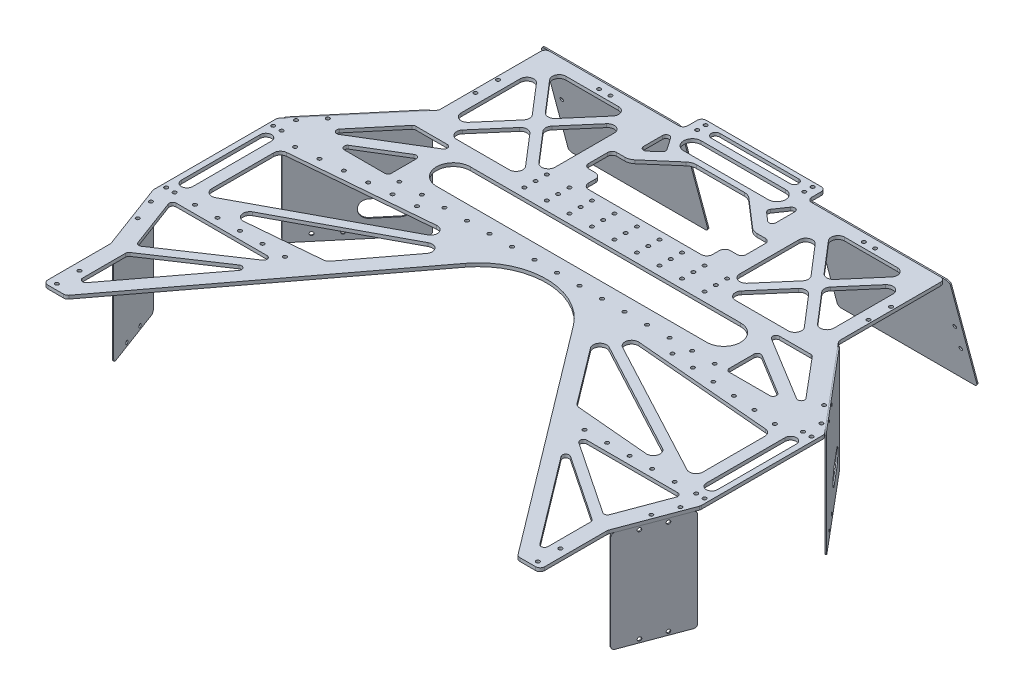
from build123d import *

# Parameters (mm, degrees)
SKETCH_1_R           = 1.6
EXTRUDE_1_DEPTH      = 3
SKETCH_2_W           = 60
SKETCH_2_H           = 90
SKETCH_2_R           = 1.6
EXTRUDE_2_DEPTH      = 1
SKETCH_3_W           = 95
SKETCH_3_H           = 96
SKETCH_3_R           = 1.6
EXTRUDE_3_DEPTH      = 1
EXTRUDE_5_DEPTH      = 4
EXTRUDE_5_DEPTH_BACK = 120
SKETCH_7_R           = 1.6
CUT_EXTRUDE_2_DEPTH  = 1
FILLET_1_R           = 3
FILLET_2_R           = 3
FILLET_3_R           = 3
CUT_EXTRUDE_4_DEPTH  = 10
CUT_EXTRUDE_1_DEPTH  = 10
CUT_EXTRUDE_3_DEPTH  = 10
FILLET_4_R           = 4
SKETCH_10_R          = 1.6
CUT_EXTRUDE_5_DEPTH  = 10


with BuildPart() as part:
    # 草图1 → 凸台-拉伸1 (new body)
    with BuildSketch(Plane(origin=(0, 0, 0), x_dir=(1, 0, 0), z_dir=(0, 1, 0))):
        with BuildLine():
            Line((-55, 0), (55, 0))
            Line((55, 0), (55, -16.419274896))
            Line((55, -16.419274896), (177.5, -16.419274896))
            Line((177.5, -16.419274896), (177.5, -111))
            Line((177.5, -111), (243, -189))
            Line((243, -189), (243, -299))
            Line((243, -299), (220.55, -359))
            Line((220.55, -359), (220.55, -419))
            Line((220.55, -419), (200.55, -419))
            Line((200.55, -419), (47.880319216, -216.840975791))
            ThreePointArc((47.880319216, -216.840975791), (0, -193), (-47.880319216, -216.840975791))
            Line((-47.880319216, -216.840975791), (-200.55, -419))
            Line((-200.55, -419), (-220.55, -419))
            Line((-220.55, -419), (-220.55, -359))
            Line((-220.55, -359), (-243, -299))
            Line((-243, -299), (-243, -189))
            Line((-243, -189), (-177.5, -111))
            Line((-177.5, -111), (-177.5, -16.419274896))
            Line((-177.5, -16.419274896), (-55, -16.419274896))
            Line((-55, -16.419274896), (-55, 0))
        make_face()
        with Locations(Location((47.5, -4, 0), (0, 0, 270))):
            Circle(SKETCH_1_R, mode=Mode.SUBTRACT)
        with Locations(Location((-47.5, -4, 0), (0, 0, 90))):
            Circle(SKETCH_1_R, mode=Mode.SUBTRACT)
        with Locations(Location((47.5, -11.5, 0), (0, 0, 270))):
            Circle(SKETCH_1_R, mode=Mode.SUBTRACT)
        with Locations(Location((-47.5, -11.5, 0), (0, 0, 90))):
            Circle(SKETCH_1_R, mode=Mode.SUBTRACT)
        with Locations(Location((231.5, -196.5, 0), (0, 0, 270))):
            Circle(SKETCH_1_R, mode=Mode.SUBTRACT)
        with Locations(Location((-231.5, -196.5, 0), (0, 0, 90))):
            Circle(SKETCH_1_R, mode=Mode.SUBTRACT)
        with Locations(Location((239, -196.5, 0), (0, 0, 270))):
            Circle(SKETCH_1_R, mode=Mode.SUBTRACT)
        with Locations(Location((-239, -196.5, 0), (0, 0, 90))):
            Circle(SKETCH_1_R, mode=Mode.SUBTRACT)
        with Locations(Location((231.5, -291.5, 0), (0, 0, 270))):
            Circle(SKETCH_1_R, mode=Mode.SUBTRACT)
        with Locations(Location((-231.5, -291.5, 0), (0, 0, 90))):
            Circle(SKETCH_1_R, mode=Mode.SUBTRACT)
        with Locations(Location((239, -291.5, 0), (0, 0, 270))):
            Circle(SKETCH_1_R, mode=Mode.SUBTRACT)
        with Locations(Location((-239, -291.5, 0), (0, 0, 90))):
            Circle(SKETCH_1_R, mode=Mode.SUBTRACT)
        with Locations(Location((213.55, -394, 0), (0, 0, 270))):
            Circle(SKETCH_1_R, mode=Mode.SUBTRACT)
        with Locations(Location((-213.55, -394, 0), (0, 0, 90))):
            Circle(SKETCH_1_R, mode=Mode.SUBTRACT)
        with Locations(Location((213.55, -414, 0), (0, 0, 270))):
            Circle(SKETCH_1_R, mode=Mode.SUBTRACT)
        with Locations(Location((-213.55, -414, 0), (0, 0, 90))):
            Circle(SKETCH_1_R, mode=Mode.SUBTRACT)
        with Locations(Location((234.987500732, -309, 0), (0, 0, 270))):
            Circle(SKETCH_1_R, mode=Mode.SUBTRACT)
        with Locations(Location((227.978719043, -327.731710526, 0), (0, 0, 270))):
            Circle(SKETCH_1_R, mode=Mode.SUBTRACT)
        with Locations(Location((-227.978719043, -327.731710526, 0), (0, 0, 90))):
            Circle(SKETCH_1_R, mode=Mode.SUBTRACT)
        with Locations(Location((-234.987500732, -309, 0), (0, 0, 90))):
            Circle(SKETCH_1_R, mode=Mode.SUBTRACT)
        with Locations(Location((220.342791881, -166.683968756, 0), (0, 0, 270))):
            Circle(SKETCH_1_R, mode=Mode.SUBTRACT)
        with Locations(Location((233.204330939, -182, 0), (0, 0, 270))):
            Circle(SKETCH_1_R, mode=Mode.SUBTRACT)
        with Locations(Location((-233.204330939, -182, 0), (0, 0, 90))):
            Circle(SKETCH_1_R, mode=Mode.SUBTRACT)
        with Locations(Location((-220.342791881, -166.683968756, 0), (0, 0, 90))):
            Circle(SKETCH_1_R, mode=Mode.SUBTRACT)
        with Locations(Location((112.5, -23.615427319, 0), (0, 0, 270))):
            Circle(SKETCH_1_R, mode=Mode.SUBTRACT)
        with Locations(Location((122.5, -23.615427319, 0), (0, 0, 270))):
            Circle(SKETCH_1_R, mode=Mode.SUBTRACT)
        with Locations(Location((-122.5, -23.615427319, 0), (0, 0, 90))):
            Circle(SKETCH_1_R, mode=Mode.SUBTRACT)
        with Locations(Location((-112.5, -23.615427319, 0), (0, 0, 90))):
            Circle(SKETCH_1_R, mode=Mode.SUBTRACT)
        with Locations(Location((174.5, -61.419274896, 0), (0, 0, 270))):
            Circle(SKETCH_1_R, mode=Mode.SUBTRACT)
        with Locations(Location((174.5, -81.419274896, 0), (0, 0, 270))):
            Circle(SKETCH_1_R, mode=Mode.SUBTRACT)
        with Locations(Location((-174.5, -81.419274896, 0), (0, 0, 90))):
            Circle(SKETCH_1_R, mode=Mode.SUBTRACT)
        with Locations(Location((-174.5, -61.419274896, 0), (0, 0, 90))):
            Circle(SKETCH_1_R, mode=Mode.SUBTRACT)
    extrude(amount=EXTRUDE_1_DEPTH)

    # 草图4 → 切除-拉伸1 (cut)
    with BuildSketch(Plane(origin=(0, 3, 0), x_dir=(1, 0, 0), z_dir=(0, 1, 0))):
        with BuildLine():
            Line((-50, -105.5), (50, -105.5))
            ThreePointArc((50, -105.5), (53.535533906, -104.035533906), (55, -100.5))
            Line((55, -100.5), (55, -94.5))
            ThreePointArc((55, -94.5), (56.464466094, -90.964466094), (60, -89.5))
            Line((60, -89.5), (66, -89.5))
            ThreePointArc((66, -89.5), (68.828427125, -88.328427125), (70, -85.5))
            Line((70, -85.5), (70, -68.5))
            ThreePointArc((70, -68.5), (68.828427125, -65.671572875), (66, -64.5))
            Line((66, -64.5), (58.730333263, -64.5))
            ThreePointArc((58.730333263, -64.5), (55.235258748, -63.869335843), (52.181027878, -62.056890828))
            Line((52.181027878, -62.056890828), (27.818972122, -40.943109172))
            ThreePointArc((27.818972122, -40.943109172), (24.764741252, -39.130664157), (21.269666737, -38.5))
            Line((21.269666737, -38.5), (-21.269666737, -38.5))
            ThreePointArc((-21.269666737, -38.5), (-24.764741252, -39.130664157), (-27.818972122, -40.943109172))
            Line((-27.818972122, -40.943109172), (-52.181027878, -62.056890828))
            ThreePointArc((-52.181027878, -62.056890828), (-55.235258748, -63.869335843), (-58.730333263, -64.5))
            Line((-58.730333263, -64.5), (-66, -64.5))
            ThreePointArc((-66, -64.5), (-68.828427125, -65.671572875), (-70, -68.5))
            Line((-70, -68.5), (-70, -85.5))
            ThreePointArc((-70, -85.5), (-68.828427125, -88.328427125), (-66, -89.5))
            Line((-66, -89.5), (-60, -89.5))
            ThreePointArc((-60, -89.5), (-56.464466094, -90.964466094), (-55, -94.5))
            Line((-55, -94.5), (-55, -100.5))
            ThreePointArc((-55, -100.5), (-53.535533906, -104.035533906), (-50, -105.5))
        make_face()
    extrude(amount=-CUT_EXTRUDE_1_DEPTH, mode=Mode.SUBTRACT)

    # 草图8 → 切除-拉伸3 (cut)
    with BuildSketch(Plane(origin=(0, 3, 0), x_dir=(1, 0, 0), z_dir=(0, 1, 0))):
        with BuildLine():
            Line((238, -209), (238, -279))
            ThreePointArc((238, -279), (233, -284), (228, -279))
            Line((228, -279), (228, -209))
            ThreePointArc((228, -209), (233, -204), (238, -209))
        make_face()
        with BuildLine():
            Line((-238, -209), (-238, -279))
            ThreePointArc((-238, -279), (-233, -284), (-228, -279))
            Line((-228, -279), (-228, -209))
            ThreePointArc((-228, -209), (-233, -204), (-238, -209))
        make_face()
        with BuildLine():
            Line((206.55, -398.082426617), (206.55, -360.028410476))
            ThreePointArc((206.55, -360.028410476), (206.196356405, -358.615329524), (205.21880148, -357.535399923))
            Line((205.21880148, -357.535399923), (147.100440737, -318.631430456))
            ThreePointArc((147.100440737, -318.631430456), (143.250801795, -319.064356553), (143.037623296, -322.932392219))
            Line((143.037623296, -322.932392219), (201.155984039, -399.890377828))
            ThreePointArc((201.155984039, -399.890377828), (204.503402359, -400.926899141), (206.55, -398.082426617))
        make_face()
        with BuildLine():
            Line((-206.55, -398.082426617), (-206.55, -360.028410476))
            ThreePointArc((-206.55, -360.028410476), (-206.196356405, -358.615329524), (-205.21880148, -357.535399923))
            Line((-205.21880148, -357.535399923), (-147.100440737, -318.631430456))
            ThreePointArc((-147.100440737, -318.631430456), (-143.250801795, -319.064356553), (-143.037623296, -322.932392219))
            Line((-143.037623296, -322.932392219), (-201.155984039, -399.890377828))
            ThreePointArc((-201.155984039, -399.890377828), (-204.503402359, -400.926899141), (-206.55, -398.082426617))
        make_face()
        with BuildLine():
            Line((209.318721671, -346.213334716), (225.468509872, -303.051317253))
            ThreePointArc((225.468509872, -303.051317253), (225.123905596, -300.290314614), (222.658753293, -299))
            Line((222.658753293, -299), (142.029537012, -299))
            ThreePointArc((142.029537012, -299), (139.159081329, -301.127942565), (140.360735532, -304.493010553))
            Line((140.360735532, -304.493010553), (204.840163612, -347.655028016))
            ThreePointArc((204.840163612, -347.655028016), (207.428239005, -348.017702227), (209.318721671, -346.213334716))
        make_face()
        with BuildLine():
            Line((-209.318721671, -346.213334716), (-225.468509872, -303.051317253))
            ThreePointArc((-225.468509872, -303.051317253), (-225.123905596, -300.290314614), (-222.658753293, -299))
            Line((-222.658753293, -299), (-142.029537012, -299))
            ThreePointArc((-142.029537012, -299), (-139.159081329, -301.127942565), (-140.360735532, -304.493010553))
            Line((-140.360735532, -304.493010553), (-204.840163612, -347.655028016))
            ThreePointArc((-204.840163612, -347.655028016), (-207.428239005, -348.017702227), (-209.318721671, -346.213334716))
        make_face()
        with BuildLine():
            Line((-35, -4), (35, -4))
            ThreePointArc((35, -4), (38.75, -7.75), (35, -11.5))
            Line((35, -11.5), (-35, -11.5))
            ThreePointArc((-35, -11.5), (-38.75, -7.75), (-35, -4))
        make_face()
        with BuildLine():
            Line((-37.5, -18), (37.5, -18))
            ThreePointArc((37.5, -18), (45.25, -25.75), (37.5, -33.5))
            Line((37.5, -33.5), (-37.5, -33.5))
            ThreePointArc((-37.5, -33.5), (-45.25, -25.75), (-37.5, -18))
        make_face()
        with BuildLine():
            Line((53.262700552, -29.327417709), (45.9577168, -39.893024035))
            ThreePointArc((45.9577168, -39.893024035), (45.449090517, -41.975800238), (46.460557895, -43.866194682))
            Line((46.460557895, -43.866194682), (53.765541647, -50.1971806))
            ThreePointArc((53.765541647, -50.1971806), (56.976452269, -50.659066892), (58.730333263, -47.930113352))
            Line((58.730333263, -47.930113352), (58.730333263, -31.033521107))
            ThreePointArc((58.730333263, -31.033521107), (56.623950034, -28.169703888), (53.262700552, -29.327417709))
        make_face()
        with BuildLine():
            Line((-53.262700552, -29.327417709), (-45.9577168, -39.893024035))
            ThreePointArc((-45.9577168, -39.893024035), (-45.449090517, -41.975800238), (-46.460557895, -43.866194682))
            Line((-46.460557895, -43.866194682), (-53.765541647, -50.1971806))
            ThreePointArc((-53.765541647, -50.1971806), (-56.976452269, -50.659066892), (-58.730333263, -47.930113352))
            Line((-58.730333263, -47.930113352), (-58.730333263, -31.033521107))
            ThreePointArc((-58.730333263, -31.033521107), (-56.623950034, -28.169703888), (-53.262700552, -29.327417709))
        make_face()
        with BuildLine():
            Line((72.677992184, -226.446337249), (109.351647332, -275.008109966))
            ThreePointArc((109.351647332, -275.008109966), (111.233567595, -276.641447016), (113.616744797, -277.369375734))
            Line((113.616744797, -277.369375734), (178.57816518, -283.052763583))
            ThreePointArc((178.57816518, -283.052763583), (184.852678678, -278.784202584), (181.926242178, -271.7823384))
            Line((181.926242178, -271.7823384), (80.291166647, -217.537177833))
            ThreePointArc((80.291166647, -217.537177833), (72.90460831, -218.932552589), (72.677992184, -226.446337249))
        make_face()
        with BuildLine():
            Line((212.51341094, -211.030519833), (89.80099749, -200.491550029))
            ThreePointArc((89.80099749, -200.491550029), (83.534648252, -204.765518849), (86.462444008, -211.762800768))
            Line((86.462444008, -211.762800768), (209.174857458, -277.257459343))
            ThreePointArc((209.174857458, -277.257459343), (215.086190593, -277.109630185), (218, -271.964202348))
            Line((218, -271.964202348), (218, -217.008513577))
            ThreePointArc((218, -217.008513577), (216.420433556, -212.951449715), (212.51341094, -211.030519833))
        make_face()
        with BuildLine():
            Line((-120, -140.5), (120, -140.5))
            ThreePointArc((120, -140.5), (135, -155.5), (120, -170.5))
            Line((120, -170.5), (-120, -170.5))
            ThreePointArc((-120, -170.5), (-135, -155.5), (-120, -140.5))
        make_face()
        with BuildLine():
            Line((100.350753729, -125.5), (147.149246271, -125.5))
            ThreePointArc((147.149246271, -125.5), (152.602461969, -122.002486473), (151.698112445, -115.587479517))
            Line((151.698112445, -115.587479517), (128.298866174, -88.382499937))
            ThreePointArc((128.298866174, -88.382499937), (123.75, -86.29502042), (119.201133826, -88.382499937))
            Line((119.201133826, -88.382499937), (95.801887555, -115.587479517))
            ThreePointArc((95.801887555, -115.587479517), (94.897538031, -122.002486473), (100.350753729, -125.5))
        make_face()
        with BuildLine():
            Line((82, -103.188756541), (82, -50.730518355))
            ThreePointArc((82, -50.730518355), (85.913519356, -45.1049874), (92.548866174, -46.817997872))
            Line((92.548866174, -46.817997872), (115.108766112, -73.047116965))
            ThreePointArc((115.108766112, -73.047116965), (116.559899938, -76.959637448), (115.108766112, -80.872157931))
            Line((115.108766112, -80.872157931), (92.548866174, -107.101277025))
            ThreePointArc((92.548866174, -107.101277025), (85.913519356, -108.814287496), (82, -103.188756541))
        make_face()
        with BuildLine():
            Line((100.350753729, -28.419274896), (147.149246271, -28.419274896))
            ThreePointArc((147.149246271, -28.419274896), (152.602461969, -31.916788423), (151.698112445, -38.331795379))
            Line((151.698112445, -38.331795379), (128.298866174, -65.536774959))
            ThreePointArc((128.298866174, -65.536774959), (123.75, -67.624254476), (119.201133826, -65.536774959))
            Line((119.201133826, -65.536774959), (95.801887555, -38.331795379))
            ThreePointArc((95.801887555, -38.331795379), (94.897538031, -31.916788423), (100.350753729, -28.419274896))
        make_face()
        with BuildLine():
            Line((165.5, -103.188756541), (165.5, -50.730518355))
            ThreePointArc((165.5, -50.730518355), (161.586480644, -45.1049874), (154.951133826, -46.817997872))
            Line((154.951133826, -46.817997872), (132.391233888, -73.047116965))
            ThreePointArc((132.391233888, -73.047116965), (130.940100062, -76.959637448), (132.391233888, -80.872157931))
            Line((132.391233888, -80.872157931), (154.951133826, -107.101277025))
            ThreePointArc((154.951133826, -107.101277025), (161.586480644, -108.814287496), (165.5, -103.188756541))
        make_face()
        with BuildLine():
            Line((-132.391233888, -73.047116965), (-154.951133826, -46.817997872))
            ThreePointArc((-154.951133826, -46.817997872), (-161.586480644, -45.1049874), (-165.5, -50.730518355))
            Line((-165.5, -50.730518355), (-165.5, -103.188756541))
            ThreePointArc((-165.5, -103.188756541), (-161.586480644, -108.814287496), (-154.951133826, -107.101277025))
            Line((-154.951133826, -107.101277025), (-132.391233888, -80.872157931))
            ThreePointArc((-132.391233888, -80.872157931), (-130.940100062, -76.959637448), (-132.391233888, -73.047116965))
        make_face()
        with BuildLine():
            Line((-128.298866174, -88.382499937), (-151.698112445, -115.587479517))
            ThreePointArc((-151.698112445, -115.587479517), (-152.602461969, -122.002486473), (-147.149246271, -125.5))
            Line((-147.149246271, -125.5), (-100.350753729, -125.5))
            ThreePointArc((-100.350753729, -125.5), (-94.897538031, -122.002486473), (-95.801887555, -115.587479517))
            Line((-95.801887555, -115.587479517), (-119.201133826, -88.382499937))
            ThreePointArc((-119.201133826, -88.382499937), (-123.75, -86.29502042), (-128.298866174, -88.382499937))
        make_face()
        with BuildLine():
            Line((-128.298866174, -65.536774959), (-151.698112445, -38.331795379))
            ThreePointArc((-151.698112445, -38.331795379), (-152.602461969, -31.916788423), (-147.149246271, -28.419274896))
            Line((-147.149246271, -28.419274896), (-100.350753729, -28.419274896))
            ThreePointArc((-100.350753729, -28.419274896), (-94.897538031, -31.916788423), (-95.801887555, -38.331795379))
            Line((-95.801887555, -38.331795379), (-119.201133826, -65.536774959))
            ThreePointArc((-119.201133826, -65.536774959), (-123.75, -67.624254476), (-128.298866174, -65.536774959))
        make_face()
        with BuildLine():
            Line((-92.548866174, -107.101277025), (-115.108766112, -80.872157931))
            ThreePointArc((-115.108766112, -80.872157931), (-116.559899938, -76.959637448), (-115.108766112, -73.047116965))
            Line((-115.108766112, -73.047116965), (-92.548866174, -46.817997872))
            ThreePointArc((-92.548866174, -46.817997872), (-85.913519356, -45.1049874), (-82, -50.730518355))
            Line((-82, -50.730518355), (-82, -103.188756541))
            ThreePointArc((-82, -103.188756541), (-85.913519356, -108.814287496), (-92.548866174, -107.101277025))
        make_face()
        with BuildLine():
            Line((-218, -217.008513577), (-218, -271.964202348))
            ThreePointArc((-218, -271.964202348), (-215.086190593, -277.109630185), (-209.174857458, -277.257459343))
            Line((-209.174857458, -277.257459343), (-86.462444008, -211.762800768))
            ThreePointArc((-86.462444008, -211.762800768), (-83.534648252, -204.765518849), (-89.80099749, -200.491550029))
            Line((-89.80099749, -200.491550029), (-212.51341094, -211.030519833))
            ThreePointArc((-212.51341094, -211.030519833), (-216.420433556, -212.951449715), (-218, -217.008513577))
        make_face()
        with BuildLine():
            Line((-80.291166647, -217.537177833), (-181.926242178, -271.7823384))
            ThreePointArc((-181.926242178, -271.7823384), (-184.852678678, -278.784202584), (-178.57816518, -283.052763583))
            Line((-178.57816518, -283.052763583), (-113.616744797, -277.369375734))
            ThreePointArc((-113.616744797, -277.369375734), (-111.233567595, -276.641447016), (-109.351647332, -275.008109966))
            Line((-109.351647332, -275.008109966), (-72.677992184, -226.446337249))
            ThreePointArc((-72.677992184, -226.446337249), (-72.90460831, -218.932552589), (-80.291166647, -217.537177833))
        make_face()
        with BuildLine():
            Line((-207.013861715, -169.471635843), (-177.706082625, -134.570769141))
            ThreePointArc((-177.706082625, -134.570769141), (-176.676019137, -133.780837208), (-175.408677939, -133.5))
            Line((-175.408677939, -133.5), (-147.487984577, -133.5))
            ThreePointArc((-147.487984577, -133.5), (-144.599746368, -135.68877867), (-145.925984283, -139.061279969))
            Line((-145.925984283, -139.061279969), (-203.154456734, -173.962146671))
            ThreePointArc((-203.154456734, -173.962146671), (-206.991622248, -173.356275411), (-207.013861715, -169.471635843))
        make_face()
        with BuildLine():
            Line((207.013861715, -169.471635843), (177.706082625, -134.570769141))
            ThreePointArc((177.706082625, -134.570769141), (176.676019137, -133.780837208), (175.408677939, -133.5))
            Line((175.408677939, -133.5), (147.487984577, -133.5))
            ThreePointArc((147.487984577, -133.5), (144.599746368, -135.68877867), (145.925984283, -139.061279969))
            Line((145.925984283, -139.061279969), (203.154456734, -173.962146671))
            ThreePointArc((203.154456734, -173.962146671), (206.991622248, -173.356275411), (207.013861715, -169.471635843))
        make_face()
        with BuildLine():
            Line((-154.562000294, -156.040860518), (-190.468875058, -177.938720031))
            ThreePointArc((-190.468875058, -177.938720031), (-191.795112974, -181.31122133), (-188.906874764, -183.5))
            Line((-188.906874764, -183.5), (-153, -183.5))
            ThreePointArc((-153, -183.5), (-150.878679656, -182.621320344), (-150, -180.5))
            Line((-150, -180.5), (-150, -158.602140488))
            ThreePointArc((-150, -158.602140488), (-151.53132728, -155.986227561), (-154.562000294, -156.040860518))
        make_face()
        with BuildLine():
            Line((154.562000294, -156.040860518), (190.468875058, -177.938720031))
            ThreePointArc((190.468875058, -177.938720031), (191.795112974, -181.31122133), (188.906874764, -183.5))
            Line((188.906874764, -183.5), (153, -183.5))
            ThreePointArc((153, -183.5), (150.878679656, -182.621320344), (150, -180.5))
            Line((150, -180.5), (150, -158.602140488))
            ThreePointArc((150, -158.602140488), (151.53132728, -155.986227561), (154.562000294, -156.040860518))
        make_face()
    extrude(amount=-CUT_EXTRUDE_3_DEPTH, mode=Mode.SUBTRACT)

    # 圆角4
    fillet_4_edges = [part.edges().sort_by_distance(p)[0] for p in [
        (-55, 1.5, 16.419274896),
        (-55, 1.5, 0),
        (55, 1.5, 0),
        (55, 1.5, 16.419274896),
        (177.5, 1.5, 16.419274896),
        (177.5, 1.5, 111),
        (243, 1.5, 189),
        (243, 1.5, 299),
        (220.55, 1.5, 359),
        (220.55, 1.5, 419),
        (200.55, 1.5, 419),
        (-200.55, 1.5, 419),
        (-220.55, 1.5, 419),
        (-220.55, 1.5, 359),
        (-243, 1.5, 299),
        (-243, 1.5, 189),
        (-177.5, 1.5, 111),
        (-177.5, 1.5, 16.419274896),
    ]]
    fillet(fillet_4_edges, radius=FILLET_4_R)

    # 草图10 → 切除-拉伸5 (cut)
    with BuildSketch(Plane(origin=(0, 3, 0), x_dir=(1, 0, 0), z_dir=(0, 1, 0))):
        with Locations(Location((-80, -132.5, 0), (0, 0, 270))):
            Circle(SKETCH_10_R)
        with Locations(Location((-60, -132.5, 0), (0, 0, 270))):
            Circle(SKETCH_10_R)
        with Locations(Location((-40, -132.5, 0), (0, 0, 270))):
            Circle(SKETCH_10_R)
        with Locations(Location((-20, -132.5, 0), (0, 0, 270))):
            Circle(SKETCH_10_R)
        with Locations(Location((0, -132.5, 0), (0, 0, 270))):
            Circle(SKETCH_10_R)
        with Locations(Location((20, -132.5, 0), (0, 0, 270))):
            Circle(SKETCH_10_R)
        with Locations(Location((40, -132.5, 0), (0, 0, 270))):
            Circle(SKETCH_10_R)
        with Locations(Location((60, -132.5, 0), (0, 0, 270))):
            Circle(SKETCH_10_R)
        with Locations(Location((80, -132.5, 0), (0, 0, 270))):
            Circle(SKETCH_10_R)
        with Locations(Location((-80, -122.5, 0), (0, 0, 270))):
            Circle(SKETCH_10_R)
        with Locations(Location((-60, -122.5, 0), (0, 0, 270))):
            Circle(SKETCH_10_R)
        with Locations(Location((-40, -122.5, 0), (0, 0, 270))):
            Circle(SKETCH_10_R)
        with Locations(Location((-20, -122.5, 0), (0, 0, 270))):
            Circle(SKETCH_10_R)
        with Locations(Location((0, -122.5, 0), (0, 0, 270))):
            Circle(SKETCH_10_R)
        with Locations(Location((20, -122.5, 0), (0, 0, 270))):
            Circle(SKETCH_10_R)
        with Locations(Location((40, -122.5, 0), (0, 0, 270))):
            Circle(SKETCH_10_R)
        with Locations(Location((60, -122.5, 0), (0, 0, 270))):
            Circle(SKETCH_10_R)
        with Locations(Location((80, -122.5, 0), (0, 0, 270))):
            Circle(SKETCH_10_R)
        with Locations(Location((-80, -112.5, 0), (0, 0, 270))):
            Circle(SKETCH_10_R)
        with Locations(Location((-60, -112.5, 0), (0, 0, 270))):
            Circle(SKETCH_10_R)
        with Locations(Location((-40, -112.5, 0), (0, 0, 270))):
            Circle(SKETCH_10_R)
        with Locations(Location((-20, -112.5, 0), (0, 0, 270))):
            Circle(SKETCH_10_R)
        with Locations(Location((0, -112.5, 0), (0, 0, 270))):
            Circle(SKETCH_10_R)
        with Locations(Location((20, -112.5, 0), (0, 0, 270))):
            Circle(SKETCH_10_R)
        with Locations(Location((40, -112.5, 0), (0, 0, 270))):
            Circle(SKETCH_10_R)
        with Locations(Location((60, -112.5, 0), (0, 0, 270))):
            Circle(SKETCH_10_R)
        with Locations(Location((80, -112.5, 0), (0, 0, 270))):
            Circle(SKETCH_10_R)
        with Locations(Location((-140, -183.5, 0), (0, 0, 270))):
            Circle(SKETCH_10_R)
        with Locations(Location((-120, -183.5, 0), (0, 0, 270))):
            Circle(SKETCH_10_R)
        with Locations(Location((-100, -183.5, 0), (0, 0, 270))):
            Circle(SKETCH_10_R)
        with Locations(Location((-80, -183.5, 0), (0, 0, 270))):
            Circle(SKETCH_10_R)
        with Locations(Location((-60, -183.5, 0), (0, 0, 270))):
            Circle(SKETCH_10_R)
        with Locations(Location((-40, -183.5, 0), (0, 0, 270))):
            Circle(SKETCH_10_R)
        with Locations(Location((-20, -183.5, 0), (0, 0, 270))):
            Circle(SKETCH_10_R)
        with Locations(Location((0, -183.5, 0), (0, 0, 270))):
            Circle(SKETCH_10_R)
        with Locations(Location((20, -183.5, 0), (0, 0, 270))):
            Circle(SKETCH_10_R)
        with Locations(Location((40, -183.5, 0), (0, 0, 270))):
            Circle(SKETCH_10_R)
        with Locations(Location((60, -183.5, 0), (0, 0, 270))):
            Circle(SKETCH_10_R)
        with Locations(Location((80, -183.5, 0), (0, 0, 270))):
            Circle(SKETCH_10_R)
        with Locations(Location((100, -183.5, 0), (0, 0, 270))):
            Circle(SKETCH_10_R)
        with Locations(Location((120, -183.5, 0), (0, 0, 270))):
            Circle(SKETCH_10_R)
        with Locations(Location((140, -183.5, 0), (0, 0, 270))):
            Circle(SKETCH_10_R)
        with Locations(Location((-213, -292, 0), (0, 0, 270))):
            Circle(SKETCH_10_R)
        with Locations(Location((-193, -292, 0), (0, 0, 270))):
            Circle(SKETCH_10_R)
        with Locations(Location((-173, -292, 0), (0, 0, 270))):
            Circle(SKETCH_10_R)
        with Locations(Location((-153, -292, 0), (0, 0, 270))):
            Circle(SKETCH_10_R)
        with Locations(Location((-133, -292, 0), (0, 0, 270))):
            Circle(SKETCH_10_R)
        with Locations(Location((133, -292, 0), (0, 0, 270))):
            Circle(SKETCH_10_R)
        with Locations(Location((153, -292, 0), (0, 0, 270))):
            Circle(SKETCH_10_R)
        with Locations(Location((173, -292, 0), (0, 0, 270))):
            Circle(SKETCH_10_R)
        with Locations(Location((193, -292, 0), (0, 0, 270))):
            Circle(SKETCH_10_R)
        with Locations(Location((213, -292, 0), (0, 0, 270))):
            Circle(SKETCH_10_R)
        with Locations(Location((-213, -203.04286011, 0), (0, 0, 270))):
            Circle(SKETCH_10_R)
        with Locations(Location((-193.073354186, -201.331490309, 0), (0, 0, 270))):
            Circle(SKETCH_10_R)
        with Locations(Location((-173.146708372, -199.620120509, 0), (0, 0, 270))):
            Circle(SKETCH_10_R)
        with Locations(Location((-153.220062557, -197.908750708, 0), (0, 0, 270))):
            Circle(SKETCH_10_R)
        with Locations(Location((-133.293416743, -196.197380908, 0), (0, 0, 270))):
            Circle(SKETCH_10_R)
        with Locations(Location((-113.366770929, -194.486011107, 0), (0, 0, 270))):
            Circle(SKETCH_10_R)
        with Locations(Location((113.366770929, -194.486011107, 0), (0, 0, 270))):
            Circle(SKETCH_10_R)
        with Locations(Location((133.293416743, -196.197380908, 0), (0, 0, 270))):
            Circle(SKETCH_10_R)
        with Locations(Location((153.220062557, -197.908750708, 0), (0, 0, 270))):
            Circle(SKETCH_10_R)
        with Locations(Location((173.146708372, -199.620120509, 0), (0, 0, 270))):
            Circle(SKETCH_10_R)
        with Locations(Location((193.073354186, -201.331490309, 0), (0, 0, 270))):
            Circle(SKETCH_10_R)
        with Locations(Location((213, -203.04286011, 0), (0, 0, 270))):
            Circle(SKETCH_10_R)
    extrude(amount=-CUT_EXTRUDE_5_DEPTH, mode=Mode.SUBTRACT)


with BuildPart() as body_2:
    # 草图2 → 凸台-拉伸2 (new body)
    with BuildSketch(Plane(origin=(311.294401015, 0, 116.47598838), x_dir=(0.35043908442978244, 0, -0.9365855263156783), z_dir=(0.9365855263156783, 0, 0.35043908442978244))):
        with Locations((-226.882374852, -45)):
            Rectangle(SKETCH_2_W, SKETCH_2_H)
        with Locations((-237.056123023, -3)):
            Circle(SKETCH_2_R, mode=Mode.SUBTRACT)
        with Locations((-217.056123023, -3)):
            Circle(SKETCH_2_R, mode=Mode.SUBTRACT)
        with Locations(Location((-217.056123023, -87, 0), (0, 0, 180))):
            Circle(SKETCH_2_R, mode=Mode.SUBTRACT)
        with Locations(Location((-237.056123023, -87, 0), (0, 0, 180))):
            Circle(SKETCH_2_R, mode=Mode.SUBTRACT)
    extrude(amount=-EXTRUDE_2_DEPTH)

    # 圆角1
    fillet_1_edges = [body_2.edges().sort_by_distance(p)[0] for p in [
        (241.830829068, -90, 300.69795151),
        (220.804484002, -90, 356.893083089),
        (220.804484002, 0, 356.893083089),
        (241.830829068, 0, 300.69795151),
    ]]
    fillet(fillet_1_edges, radius=FILLET_1_R)


with BuildPart() as body_3:
    # 草图3 → 凸台-拉伸3 (new body)
    with BuildSketch(Plane(origin=(49.4311396, 0, -41.509482613), x_dir=(-0.6430769528780669, 0, -0.7658015622059416), z_dir=(0.7658015622059415, 0, -0.6430769528780668))):
        with Locations((-250.504194806, -45)):
            Rectangle(SKETCH_3_W, SKETCH_3_H)
        with Locations((-279.344214859, -3)):
            Circle(SKETCH_3_R, mode=Mode.SUBTRACT)
        with Locations((-259.344214859, -3)):
            Circle(SKETCH_3_R, mode=Mode.SUBTRACT)
        with Locations(Location((-259.344214859, -87, 0), (0, 0, 180))):
            Circle(SKETCH_3_R, mode=Mode.SUBTRACT)
        with Locations(Location((-279.344214859, -87, 0), (0, 0, 180))):
            Circle(SKETCH_3_R, mode=Mode.SUBTRACT)
    extrude(amount=EXTRUDE_3_DEPTH)

    # 圆角2
    fillet_2_edges = [body_3.edges().sort_by_distance(p)[0] for p in [
        (241.453669922, 3, 186.381056837),
        (180.361359399, 3, 113.629908427),
        (180.361359399, -93, 113.629908427),
        (241.453669922, -93, 186.381056837),
    ]]
    fillet(fillet_2_edges, radius=FILLET_2_R)

    # 草图9 → 切除-拉伸4 (cut)
    with BuildSketch(Plane(origin=(50.196941163, 0, -42.152559566), x_dir=(-0.6430769528780668, 0, -0.7658015622059418), z_dir=(0.7658015622059416, 0, -0.6430769528780667))):
        with BuildLine():
            Line((-243.004194806, -62.5), (-223.004194806, -62.5))
            ThreePointArc((-223.004194806, -62.5), (-215.504194806, -70), (-223.004194806, -77.5))
            Line((-223.004194806, -77.5), (-243.004194806, -77.5))
            ThreePointArc((-243.004194806, -77.5), (-250.504194806, -70), (-243.004194806, -62.5))
        make_face()
    extrude(amount=-CUT_EXTRUDE_4_DEPTH, mode=Mode.SUBTRACT)


with BuildPart() as body_4:
    # 草图6 → 凸台-拉伸5 (new, two sides: drawn at the far end of the back side and taken through both)
    with BuildSketch(Plane(origin=(177.5, 0, 0), x_dir=(0, 0, -1), z_dir=(1, 0, 0)).offset(-EXTRUDE_5_DEPTH_BACK)):
        Polygon((-16.419274896, 3), (8.5, -90), (9.465925826, -89.741180955), (-15.45334907, 3.258819045), align=None)
    extrude(amount=EXTRUDE_5_DEPTH + EXTRUDE_5_DEPTH_BACK)

    # 草图7 → 切除-拉伸2 (cut)
    with BuildSketch(Plane(origin=(0, -3.645037785, 13.603466208), x_dir=(-1, 0, 0), z_dir=(0, 0.2588190451025185, -0.965925826289069))):
        with Locations(Location((-122.5, -3.75037895, 0), (0, 0, 90))):
            Circle(SKETCH_7_R)
        with Locations(Location((-112.5, -3.75037895, 0), (0, 0, 90))):
            Circle(SKETCH_7_R)
        with Locations(Location((-174.5, -37.852601471, 0), (0, 0, 90))):
            Circle(SKETCH_7_R)
        with Locations(Location((-174.5, -57.852601471, 0), (0, 0, 90))):
            Circle(SKETCH_7_R)
    extrude(amount=-CUT_EXTRUDE_2_DEPTH, mode=Mode.SUBTRACT)

    # 圆角3
    fillet_3_edges = [body_4.edges().sort_by_distance(p)[0] for p in [
        (57.5, 3.129409523, 15.936311983),
        (57.5, -89.870590477, -8.982962913),
        (181.5, -89.870590477, -8.982962913),
        (181.5, 3.129409523, 15.936311983),
    ]]
    fillet(fillet_3_edges, radius=FILLET_3_R)


with BuildPart() as body_5:
    # 镜向1: mirrored copy
    add(body_2.part.mirror(Plane(origin=(0, 0, 0), x_dir=(0, 0, 1), z_dir=(1, 0, 0))))


with BuildPart() as body_6:
    # Mirror 1 2: mirrored copy
    add(body_3.part.mirror(Plane(origin=(0, 0, 0), x_dir=(0, 0, 1), z_dir=(1, 0, 0))))


with BuildPart() as body_7:
    # Mirror 1 3: mirrored copy
    add(body_4.part.mirror(Plane(origin=(0, 0, 0), x_dir=(0, 0, 1), z_dir=(1, 0, 0))))


solid = Compound([part.part, body_2.part, body_3.part, body_4.part, body_5.part, body_6.part, body_7.part])
